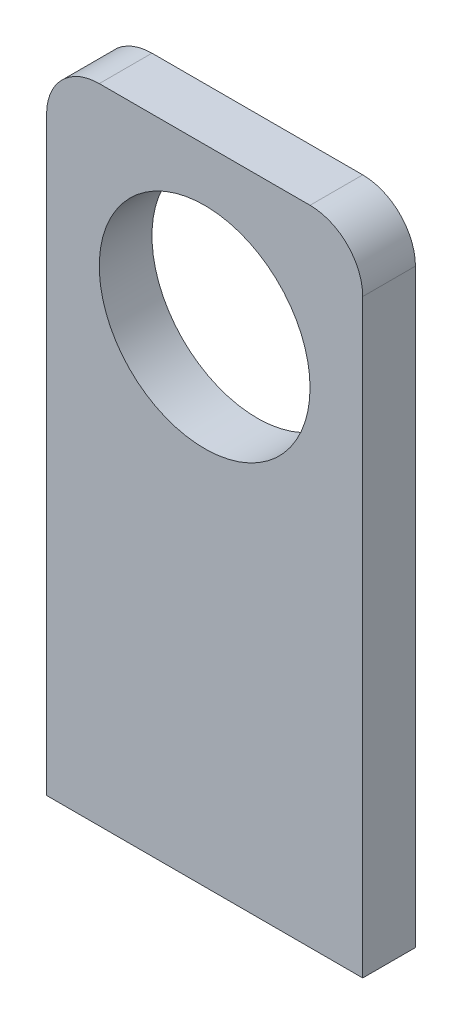
from build123d import *

# Parameters (mm, degrees)
SKETCH_1_W      = 30
SKETCH_1_H      = 61
SKETCH_1_R      = 10
EXTRUDE_1_DEPTH = 2.5
FILLET_1_R      = 5


with BuildPart() as part:
    # 草图1 → 凸台-拉伸1 (new, symmetric)
    with BuildSketch(Plane.XY):
        Rectangle(SKETCH_1_W, SKETCH_1_H)
        with Locations((0, 15.5)):
            Circle(SKETCH_1_R, mode=Mode.SUBTRACT)
    extrude(amount=EXTRUDE_1_DEPTH, both=True)

    # 圆角1
    fillet_1_edges = [part.edges().sort_by_distance(p)[0] for p in [
        (-15, 30.5, 0),
        (15, 30.5, 0),
    ]]
    fillet(fillet_1_edges, radius=FILLET_1_R)


solid = part.part
